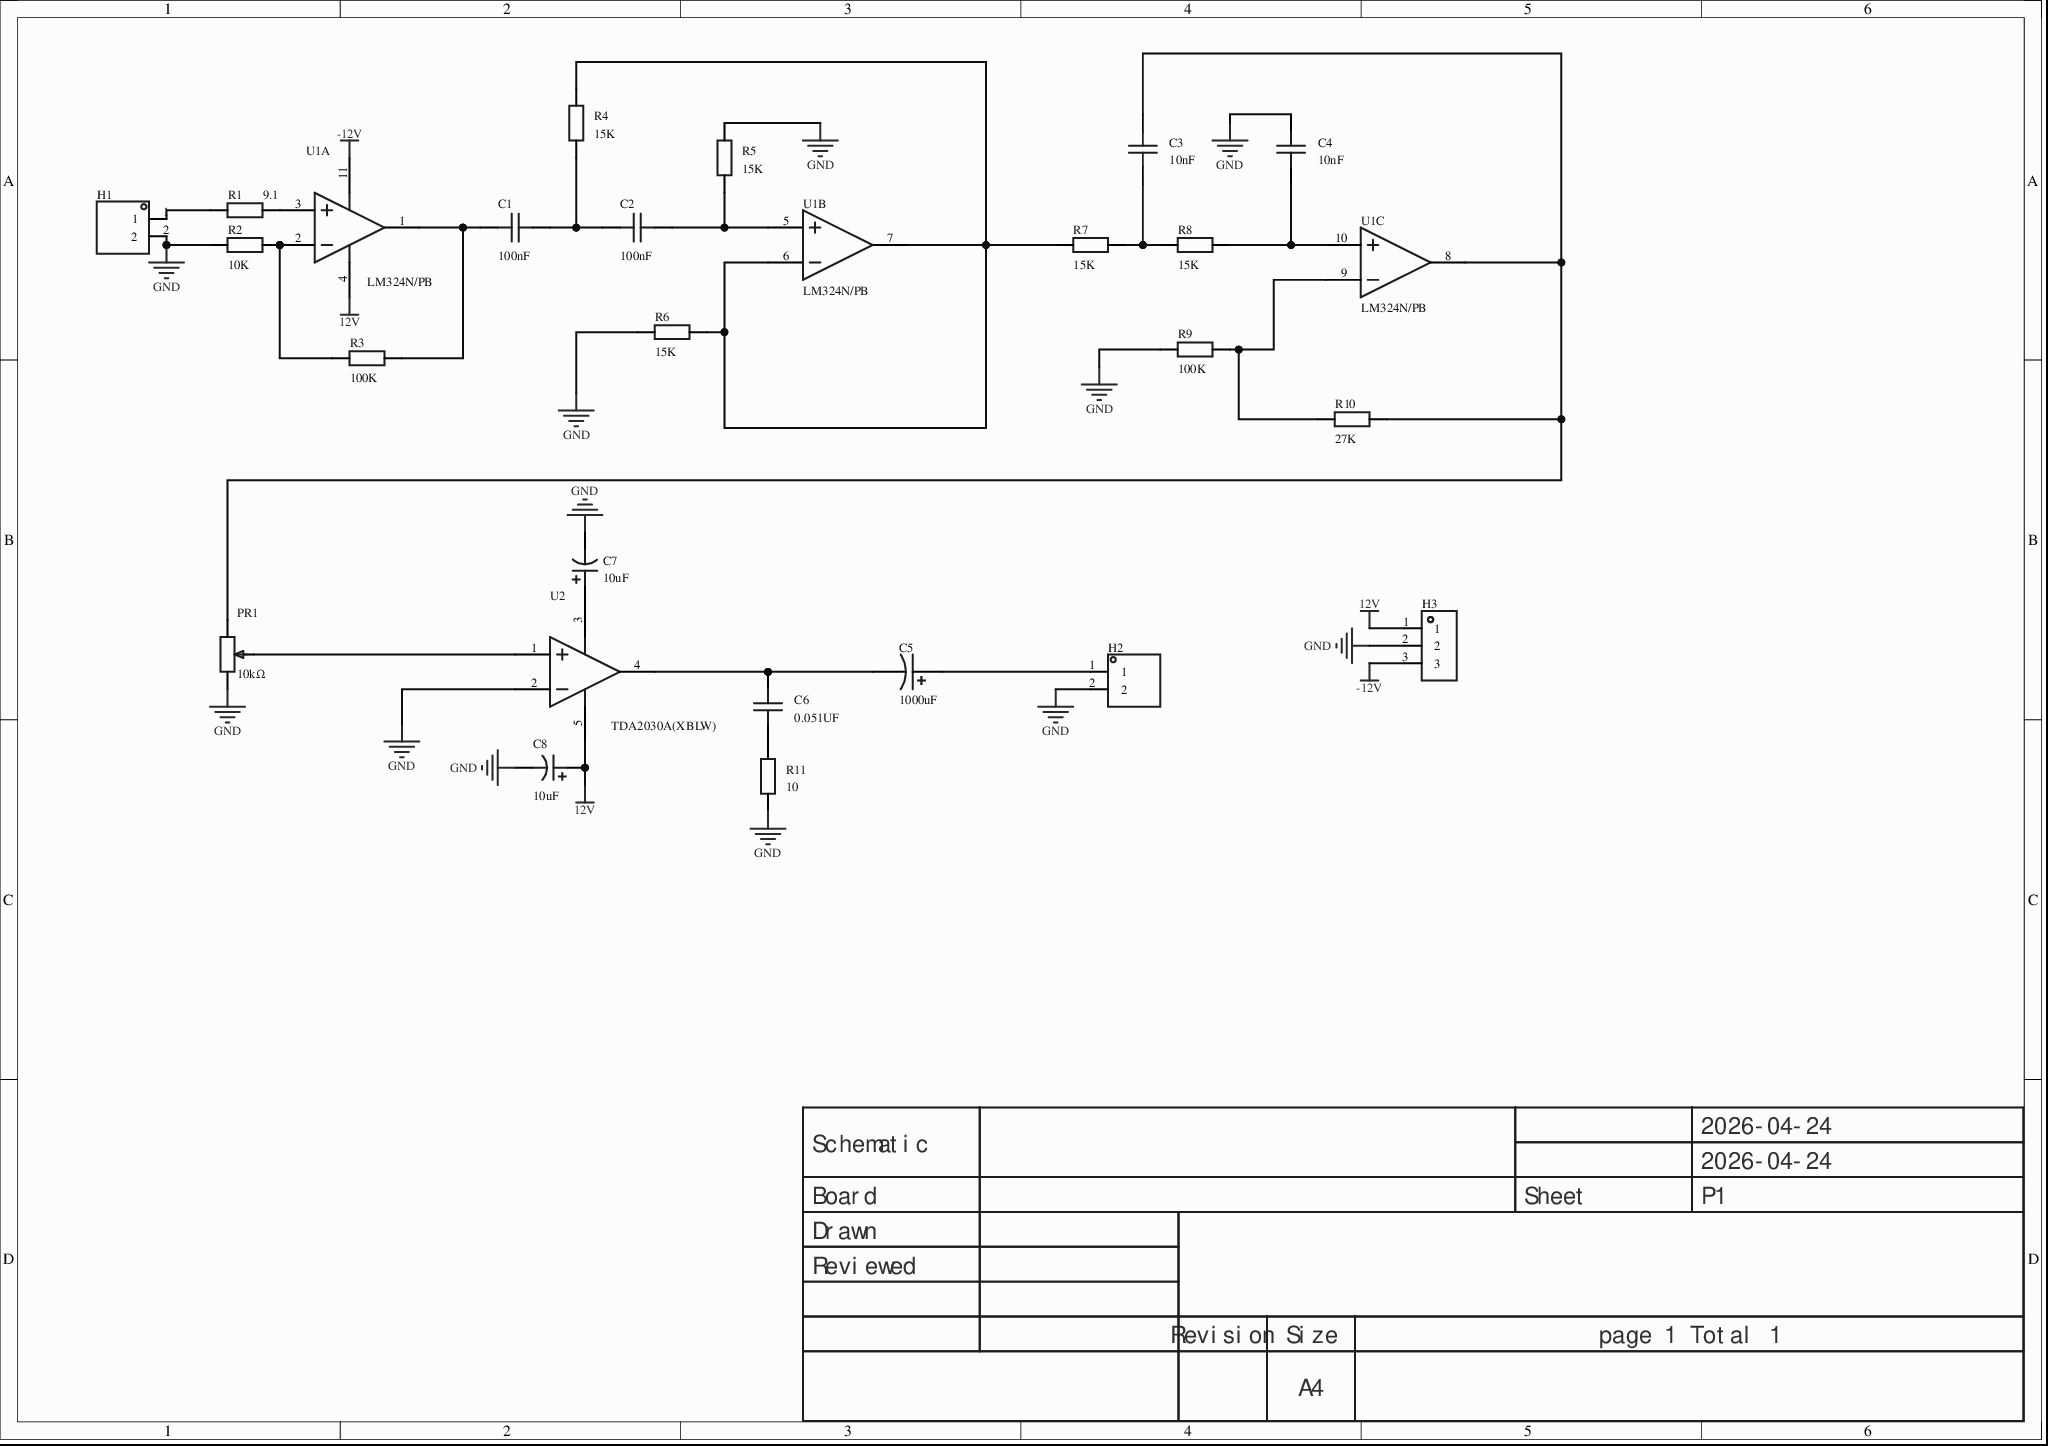
[diagram p0: MISC49872-3.schdoc]
# Altium project MISC49872-2.PrjPcb
1 sheet, 25 parts. Net scope: global (net labels, ports and power ports of the same name join across sheets).
Board file: MISC49872.pcbdoc

## Sheet MISC49872-3.schdoc
size 297 x 209 mm; Version: V1.0; @Project Name: MISC49872; @Update Date: 2026-04-24; @Create Date: 2026-04-24; @Board Name: MISC49872; @Create Time: 16:25:07; @Page Count: 1; @Page No: 1; @Schematic Name: MISC49872; @Update Time: 16:25:07; Size: A4

### Parts
C1  100nF  [C0603]
C2  100nF  [C0603]
C3  10nF  [C0603]
C4  10nF  [C0603]
C5  1000uF  [CAP-TH_BD12.5-P5.00-D0.6-FD]
C6  0.051UF  [C0603]
C7  10uF  [CAP-TH_BD5.0-P2.00-D0.8-FD-10UF50VC110GL]
C8  10uF  [CAP-TH_BD5.0-P2.00-D0.8-FD-10UF50VC110GL]
H1  (no value)  [HDR-TH_2P-P2.54-V-M-1]
H2  (no value)  [HDR-TH_2P-P2.54-V-M-1]
H3  (no value)  [HDR-TH_3P-P2.54-V-M]
PR1  10kΩ  [R_3296]
R1  9.1  [R0603]
R2  10K  [R0603]
R3  100K  [R0603]
R4  15K  [R0603]
R5  15K  [R0603]
R6  15K  [R0603]
R7  15K  [R0603]
R8  15K  [R0603]
R9  100K  [R0603]
R10  27K  [R0603]
R11  10  [R0603]
U1  LM324N/PB  [PDIP-14_L19.2-W6.6-P2.54-LS7.6-BL]  (parts A,B,C of 4)
U2  TDA2030A(XBLW)  [TO-220-5_L10.5-W15.5-P1.70-TL]

### Nets
12V: C8.1 H3.1 U1.4(V+) U2.5(VCC+)
-12V: H3.3 U1.11(GND)
GND: C4.2 C7.2 C8.2 H1.2 H2.2 H3.2 PR1.1 R2.1 R5.2 R6.2 R9.1 R11.1 U2.2(IN-)
NetC1_1: C1.1 R3.2 U1.1(OUTA)
NetC1_2: C1.2 C2.1 R4.1
NetC2_2: C2.2 R5.1 U1.5(INB+)
NetC3_1: C3.1 R7.2 R8.1
NetC3_2: C3.2 PR1.3 R10.2 U1.8(OUTC)
NetC4_1: C4.1 R8.2 U1.10(INC+)
NetC5_1: C5.1 H2.1
NetC5_2: C5.2 C6.2 U2.4(OUT)
NetC6_1: C6.1 R11.2
NetC7_1: C7.1 U2.3(VCC-)
NetH1_1: H1.1 R1.1
NetPR1_2: PR1.2 U2.1(IN+)
NetR1_2: R1.2 U1.3(INA+)
NetR2_2: R2.2 R3.1 U1.2(INA-)
NetR4_2: R4.2 R6.1 R7.1 U1.6(INB-) U1.7(OUTB)
NetR9_2: R9.2 R10.1 U1.9(INC-)

### Notes on the sheet
- 2026-04-24
- Schematic
- Board
- Sheet
- P1
- Drawn
- Reviewed
- Revision
- Size
- A4
- page 1 Total 1

### Library data of the parts
C1-C4 C6 = CAP_0603: Symbol: Capacitance; ConvertToPcb: yes; ModelId: ac125912035d415993ca9572d50418b10819f05c4eef4c71ace90d822a990e87; ModelName: C0603_L1.6-W0.8-H0.8; ModelTransform: 62.992,31.496,0,0,0,0,0,0,0; Device: CAP_0603; AddInBom: yes; Supplier Footprint: 0603; FootprintName: C0603
  C1 C2: Value: 100nF
  C3 C4: Value: 10nF
  C6: Value: 0.051UF
C5 = 50ZLJ1000M12.5X35: Capacitance:1000uF;Tolerance:±20%;Rated voltage:50V;Ripple current:2.286A@120Hz;Equivalent series resistance(ESR):-;; Manufacturer: Rubycon(红宝石); AddInBom: yes; ModelId: 968d8ff988964aab8919b46a6a737be20819f05c4eef4c71ace90d822a990e87; ModelName: CAP-TH_D12.5-H20.0-P5.00; ModelTransform: 492.5187,492.11201,0,0,0,0,0,0,-137.795; Tolerance: ±20%; Voltage Rating: 50V; Pin Spacing: 5mm; Lifetime: 10000hrs@105℃; Symbol: 50ZLJ1000M12.5X35; Device: 50ZLJ1000M12.5X35; LCSC Part Name: 1000uF ±20% 50V; SupplierPart: C1650817; ManufacturerPart: 50ZLJ1000M12.5X35; Supplier Footprint: 插件,D12.5xL35mm; JLCPCB Part Class: Extended Part; Datasheet: https://atta.szlcsc.com/upload/public/pdf/source/20210511/C1650817_FD11007E527E14F557ACD264BDA4BB64.pdf; Supplier: LCSC; ConvertToPcb: yes; FootprintName: CAP-TH_BD12.5-P5.00-D0.6-FD; Value: 1000uF; Ripple Current: 2.286A@120Hz; Equivalent Series Resistance(ESR): -; Diameter: 12.5mm; Height - Seated (Max): 35mm; Operating Temperature: -40℃~+105℃
C7 C8 = 10UF50VC110GL: Capacitance:10uF;Tolerance:±20%;Rated voltage:50V;Ripple current:120mA@100KHz;Equivalent series resistance(ESR):1.6Ω;; Manufacturer: Econd(米朗电子); AddInBom: yes; Tolerance: ±20%; Voltage Rating: 50V; Equivalent Series Resistance(ESR): 1.6Ω; Pin Spacing: 2mm; Lifetime: 5000hrs@105℃; Symbol: 10UF50VC110GL; Device: 10UF50VC110GL; LCSC Part Name: 10uF ±20% 50V; SupplierPart: C46867109; ManufacturerPart: 10UF50VC110GL; Supplier Footprint: 插件,D5xL11mm; JLCPCB Part Class: Extended Part; Datasheet: https://item.szlcsc.com/datasheet/10UF50VC110GL/49031974.html; Supplier: LCSC; ConvertToPcb: yes; FootprintName: CAP-TH_BD5.0-P2.00-D0.8-FD-10UF50VC110GL; Value: 10uF; Ripple Current: 120mA@100KHz; Diameter: 5mm; Height - Seated (Max): 11mm; Operating Temperature: -40℃~+105℃
H1 H2 = HDR-M_2.54_1x2P: Symbol: 210S-1*2P L=11.6MMGold-plated black; ConvertToPcb: yes; ModelId: 79b2e9f2d70a4d68a1b7098f27c6d4c50819f05c4eef4c71ace90d822a990e87; ModelName: HDR-M-2.54_1x2; ModelTransform: 200,100,0,0,0,0,0,0,-118.11; Device: HDR-M_2.54_1x2P; AddInBom: yes; SupplierPart: C124375; Supplier Footprint: 插件; FootprintName: HDR-TH_2P-P2.54-V-M-1
H3 = HDR-M_2.54_1x3P: AddInBom: yes; ModelId: bb473b6d38ff42a99216a4fcdbdcc4cb0819f05c4eef4c71ace90d822a990e87; ModelName: HDR-TH_3P-P2.54-M-LI-1X3P; ModelTransform: 300.03877,100,0,0,0,0,0,0,-118.11; Symbol: HDR-M_2.54_1x3P; Device: HDR-M_2.54_1x3P; ConvertToPcb: yes; FootprintName: HDR-TH_3P-P2.54-V-M; SupplierPart: C2937625; Supplier Footprint: 插件
PR1 = R_3296: ConvertToPcb: yes; ModelId: b182808559bb43bda9e7de64b64134cb0819f05c4eef4c71ace90d822a990e87; ModelName: 3296W; ModelTransform: 373.98,188.96,590.49,180,0,0,0,0,-140; Symbol: R_3296; Device: R_3296; AddInBom: yes; Supplier Footprint: 直插; FootprintName: R_3296; Value: 10kΩ
R1-R11 = Res_0603: Symbol: Resistor; ConvertToPcb: yes; ModelId: fc143cca1e79419f9cd78b61e9279f080819f05c4eef4c71ace90d822a990e87; ModelTransform: 31.8897,63.7794,0,90,0,0,0,0,0; Device: Res_0603; AddInBom: yes; Supplier Footprint: 0603; FootprintName: R0603; ModelName: R0603
  R1: Value: 9.1
  R2: Value: 10K
  R3 R9: Value: 100K
  R4-R8: Value: 15K
  R10: Value: 27K
  R11: Value: 10
U1 = LM324N/PB: Amplifier count:4;Rail-to-rail:-;Gain bandwidth product(GBW):-;Input offset voltage(Vos):2mV;Slew rate(SR):-;Input bias current(Ib):45nA;; Manufacturer: TI(德州仪器); Relevance: []; AddInBom: yes; ModelId: 08aeb3774ab0450ba412f07c9830bd710819f05c4eef4c71ace90d822a990e87; ModelTransform: 755.904,309.842,0,0,0,0,0,0,-129.921; Number of Channels: 4; Maximum Power Supply Range (Vdd-Vss): 32V; Vos - Input Offset Voltage: 2mV; Input Offset Voltage Drift(Vos TC): 7uV/℃; Ib - Input Bias Current: 45nA; Input Offset Current(Ios): 5nA; Common Mode Rejection Ratio(CMRR): 65dB; Quiescent Current: 700uA; Output Current: 40mA; Symbol: LM324N/PB; Device: LM324N/PB; LCSC Part Name: LM324N/PB; SupplierPart: C4366406; ManufacturerPart: LM324N/PB; Supplier Footprint: PDIP-14; JLCPCB Part Class: Extended Part; Datasheet: https://item.szlcsc.com/datasheet/LM324N%252FPB/4937320.html; Supplier: LCSC; ConvertToPcb: yes; FootprintName: PDIP-14_L19.2-W6.6-P2.54-LS7.6-BL; ModelName: PDIP-14_L19.2-W6.6-P2.54-LS7.6-BL; Rail to Rail: -; Gain Bandwidth Product: -; Slew Rate: -; Input Voltage Noise Density: -; Input offset current drift(Ios TC): -; Operating Temperature: 0℃~+70℃; Single supply: -; Dual Supply: -; Features: -
U2 = TDA2030A(XBLW): Amplifier type:Class AB amplifier;Speaker channels:-;Output power:25W;Quiescent current(Iq):26mA;; Manufacturer: XBLW(芯伯乐); AddInBom: yes; ModelId: 415e53c11dc24286948f39aa204ac26c0819f05c4eef4c71ace90d822a990e87; ModelName: TO-220-5_L10.2-W8.5-H14.9-P1.70; ModelTransform: 397.637,317.716,0,90,0,0,78.732,0,-137.795; Output Power: 25W; Voltage - Supply: -4.5V~25V; Total Harmonic Distortion + Noise (THD+N): 0.05%; Quiescent Current: 26mA; Signal-to-Noise Ratio: 106dB; Symbol: TDA2030A(XBLW); Device: TDA2030A(XBLW); LCSC Part Name: 18W 高保真放大器和 35W 驱动器; SupplierPart: C19267476; ManufacturerPart: TDA2030A(XBLW); Supplier Footprint: TO-220B; JLCPCB Part Class: Extended Part; Datasheet: https://item.szlcsc.com/datasheet/TDA2030A(XBLW)/20521867.html; Supplier: LCSC; ConvertToPcb: yes; FootprintName: TO-220-5_L10.5-W15.5-P1.70-TL; Class: Class AB amplifier; Speaker Channels: -; Operating Temperature: -20℃~+125℃